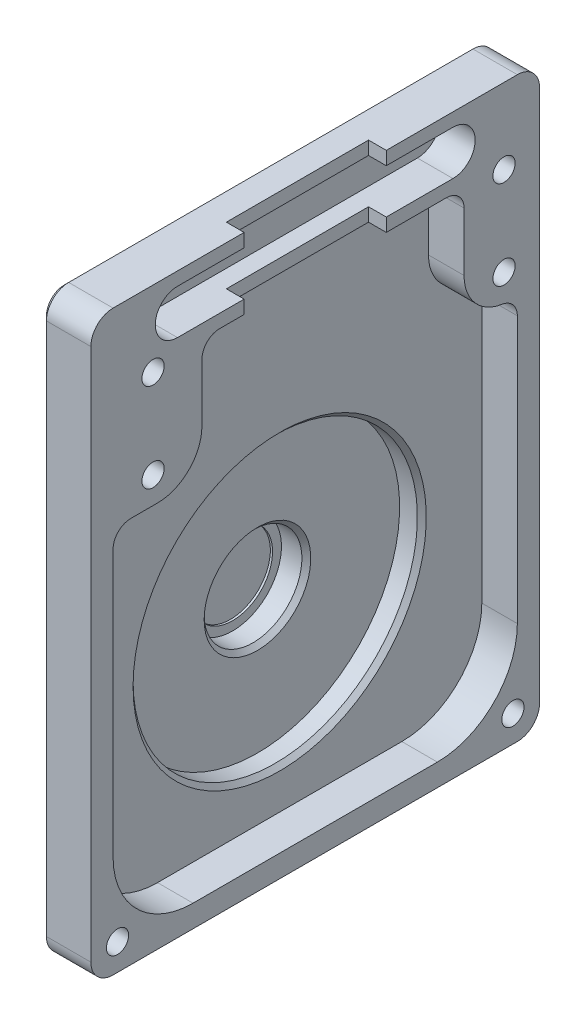
SolidWorks part; units mm, degrees
material "6061-O (GB)"
ref_plane "前视基准面" through (0, 0, 0) normal (0, 0, 1) x (1, 0, 0)
ref_plane "上视基准面" through (0, 0, 0) normal (0, 1, 0) x (1, 0, 0)
ref_plane "右视基准面" through (0, 0, 0) normal (1, 0, 0) x (0, 0, -1)
ref_plane "基准面4" through (1263, 0, 0) normal (1, 0, 0) x (0, 0, -1)
sketch "草图1" plane through (1263, 0, 0) normal (1, 0, 0) x (0, 0, -1)
  line L0 (61.5, -71.6) -> (61.5, 58.4)
  line L1 (61.5, 58.4) -> (-39.5, 58.4)
  line L2 (-39.5, 58.4) -> (-39.5, -71.6)
  line L3 (-39.5, -71.6) -> (61.5, -71.6)
extrude "凸台-拉伸1" add sketch "草图1" against normal blind 11
sketch "草图2" plane through (1263, 0, 0) normal (1, 0, 0) x (0, 0, -1)
  line L0 (44.5, 25.2564) -> (44.5, 42.4)
  line L1 (44.5, 42.4) -> (-14.5, 42.4)
  line L2 (-14.5, 42.4) -> (-14.5, 15.4)
  line L3 (-14.5, 15.4) -> (-34.5, 15.4)
  line L4 (-34.5, 15.4) -> (-34.5, -48.6)
  line L5 (-16.5, -66.6) -> (38.5, -66.6)
  line L6 (56.5, -48.6) -> (56.5, 15.4584)
  arc A0 (56.5, 15.4584) -> (44.5, 25.2564) centre (54.5, 25.2564) cw
  arc A1 (-34.5, -48.6) -> (-16.5, -66.6) centre (-16.5, -48.6) ccw
  arc A2 (38.5, -66.6) -> (56.5, -48.6) centre (38.5, -48.6) ccw
extrude "切除-拉伸1" cut sketch "草图2" against normal blind 8
sketch "草图3" plane through (1263, 0, 0) normal (1, 0, 0) x (0, 0, -1)
  line L0 (42, 55.4) -> (-20, 55.4)
  line L1 (-20, 45.4) -> (42, 45.4)
  arc A0 (-20, 55.4) -> (-20, 45.4) centre (-20, 50.4) ccw
  arc A1 (42, 45.4) -> (42, 55.4) centre (42, 50.4) ccw
extrude "切除-拉伸2" cut sketch "草图3" against normal blind 8
sketch "草图4" plane through (0, 42.4, 0) normal (0, -1, 0) x (1, 0, 0)
  line L0 (1263, -27) -> (1263, 5)
  line L1 (1263, 5) -> (1259, 5)
  line L2 (1259, 5) -> (1259, -27)
  line L3 (1259, -27) -> (1263, -27)
extrude "切除-拉伸3" cut sketch "草图4" against normal up to next
sketch "草图5" plane through (0, 58.4, 0) normal (0, 1, 0) x (-1, 0, 0)
  line L0 (-1263, 5) -> (-1263, -27)
  line L1 (-1263, -27) -> (-1259, -27)
  line L2 (-1259, -27) -> (-1259, 5)
  line L3 (-1259, 5) -> (-1263, 5)
extrude "切除-拉伸4" cut sketch "草图5" against normal up to next
sketch "草图6" plane through (1252, 0, 0) normal (-1, 0, 0) x (0, 0, 1)
  circle A0 centre (-11, -25.6) radius 36
extrude "凸台-拉伸2" add sketch "草图6" along normal blind 5
sketch "草图7" plane through (1247, 0, 0) normal (-1, 0, 0) x (0, 0, 1)
  circle A0 centre (-11, -25.6) radius 14
extrude "凸台-拉伸3" add sketch "草图7" along normal blind 4.5
sketch "草图8" plane through (1255, 0, 0) normal (1, 0, 0) x (0, 0, -1)
  circle A0 centre (11, -25.6) radius 32
extrude "切除-拉伸5" cut sketch "草图8" against normal blind 5
sketch "草图9" plane through (1250, 0, 0) normal (1, 0, 0) x (0, 0, -1)
  circle A0 centre (11, -25.6) radius 11
extrude "切除-拉伸6" cut sketch "草图9" against normal blind 5.6
sketch "草图10" plane through (1244.4, 0, 0) normal (1, 0, 0) x (0, 0, -1)
  circle A0 centre (11, -25.6) radius 9
extrude "切除-拉伸7" cut sketch "草图10" against normal blind 0.5
hole_wizard "M6 螺纹孔1" positions "草图12" profile "草图11" tap size "M6" standard "GB" end condition through all
sketch "草图12" plane through (1263, 0, 0) normal (1, 0, 0) x (0, 0, -1)
  point P0 (53.5, 41.4)
  point P1 (-25.5, 41.4)
  point P2 (-25.5, 21.4)
  point P3 (-33.5, -65.6)
  point P4 (55.5, -65.6)
  point P5 (53.5, 21.4)
sketch "草图11" plane through (1263, 41.4, -53.5) normal (0, 1, 0) x (0, 0, -1)
  line L0 (0, 0) -> (0, 20.5)
  line L1 (0, 20.5) -> (2.5, 20.5)
  line L2 (2.5, 20.5) -> (2.5, 0)
  line L5 (2.5, 0) -> (0, 0)
  line L11 (0, -6.35) -> (0, 107.95) construction
  dimension "通孔螺纹孔钻头直径" = 5
  dimension "通孔螺纹孔钻头深度" = 20.5
cosmetic thread "孔螺蚊线1" parameters "D2"=6
cosmetic thread "孔螺蚊线2" parameters "D2"=6
cosmetic thread "孔螺蚊线3" parameters "D2"=6
cosmetic thread "孔螺蚊线4" parameters "D2"=6
cosmetic thread "孔螺蚊线5" parameters "D2"=6
cosmetic thread "孔螺蚊线6" parameters "D2"=6
fillet "圆角1" radius 5 4 edges at (1257.5, 58.4, -61.5) (1257.5, -71.6, -61.5) (1257.5, 58.4, 39.5) (1257.5, -71.6, 39.5)
chamfer "倒角1" distance 1 angle 45 10 edges at (1252, -6.6, 39.5) (1252, 56.9355, 38.0355) (1252, -70.1355, 38.0355) (1252, 58.4, -11) (1252, -71.6, -11) (1252, 56.9355, -60.0355) (1252, -70.1355, -60.0355) (1252, -6.6, -61.5) (1250, -25.6, 0) (1255, -25.6, 21)
fillet "圆角2" radius 2 4 edges at (1242.5, -25.6, 3) (1247, -25.6, 3) (1252, -25.6, 25) (1247, -25.6, 25)
fillet "圆角3" radius 4 4 edges at (1259, 42.4, -44.5) (1259, 15.4584, -56.5) (1259, 42.4, 14.5) (1259, 15.4, 34.5)
fillet "圆角4" radius 10 1 edges at (1259, 15.4, 14.5)
